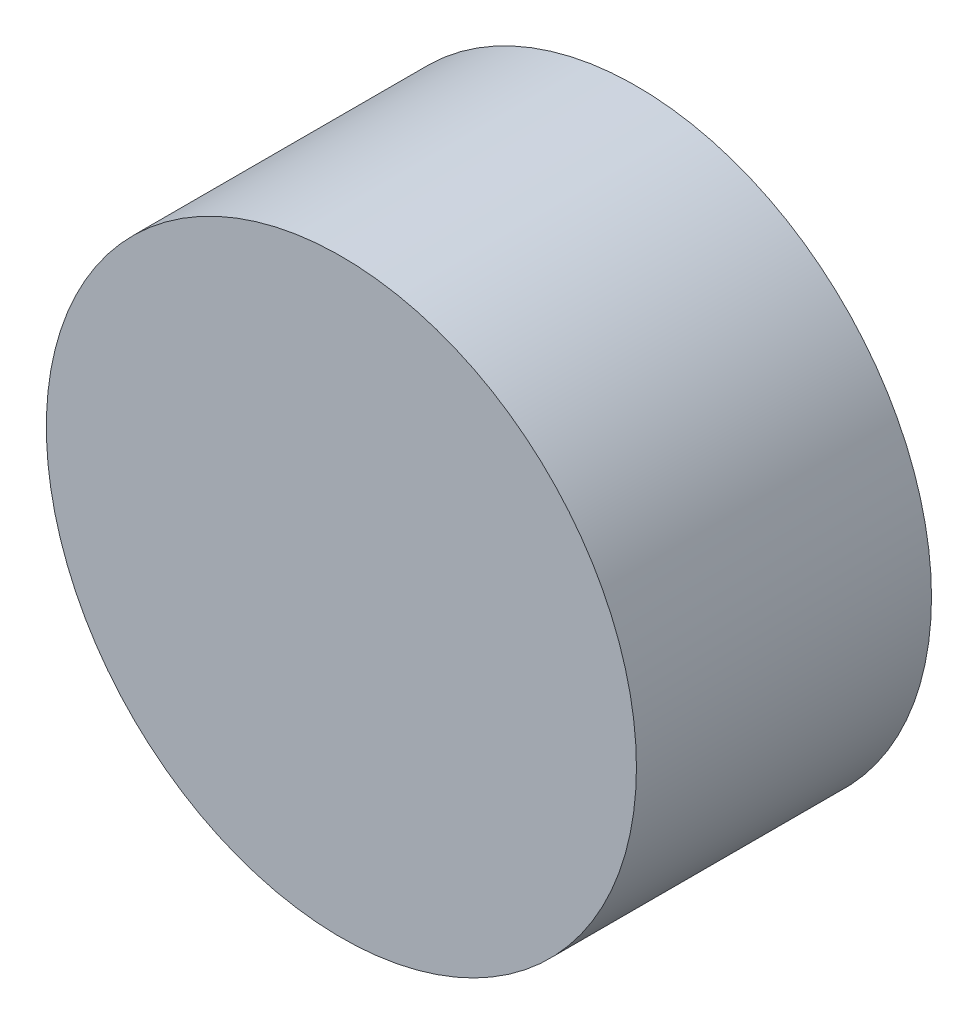
from build123d import *

# Parameters (mm, degrees)
SKETCH1_R           = 6.35
BOSS_EXTRUDE1_DEPTH = 6.35


with BuildPart() as part:
    # Sketch1 → Boss-Extrude1 (new body)
    with BuildSketch(Plane.XY):
        Circle(SKETCH1_R)
    extrude(amount=BOSS_EXTRUDE1_DEPTH)


solid = part.part
